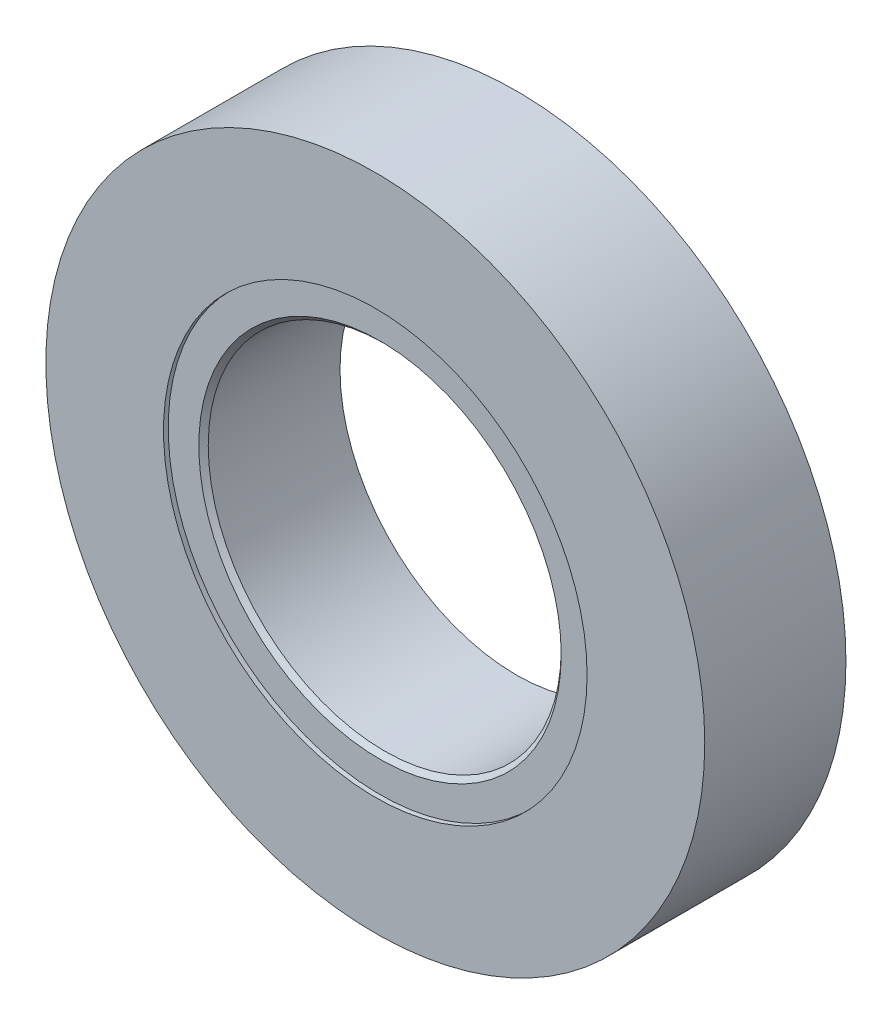
from build123d import *

# Parameters (mm, degrees)
SKETCH_1_R          = 70
SKETCH_1_R_2        = 37.5
EXTRUDE_1_DEPTH     = 30
SKETCH_2_R          = 45
CUT_EXTRUDE_1_DEPTH = 1
CHAMFER_1_SIZE      = 1


with BuildPart() as part:
    # 草图1 → 凸台-拉伸1 (new body)
    with BuildSketch(Plane.XY):
        Circle(SKETCH_1_R)
        Circle(SKETCH_1_R_2, mode=Mode.SUBTRACT)
    extrude(amount=EXTRUDE_1_DEPTH)

    # 草图2 → 切除-拉伸1 (cut)
    with BuildSketch(Plane.XY.offset(30)):
        Circle(SKETCH_2_R)
    extrude(amount=-CUT_EXTRUDE_1_DEPTH, mode=Mode.SUBTRACT)

    # 倒角1
    chamfer_1_edges = [part.edges().sort_by_distance(p)[0] for p in [
        (-37.5, 0, 29),
    ]]
    chamfer(chamfer_1_edges, length=CHAMFER_1_SIZE)


solid = part.part
